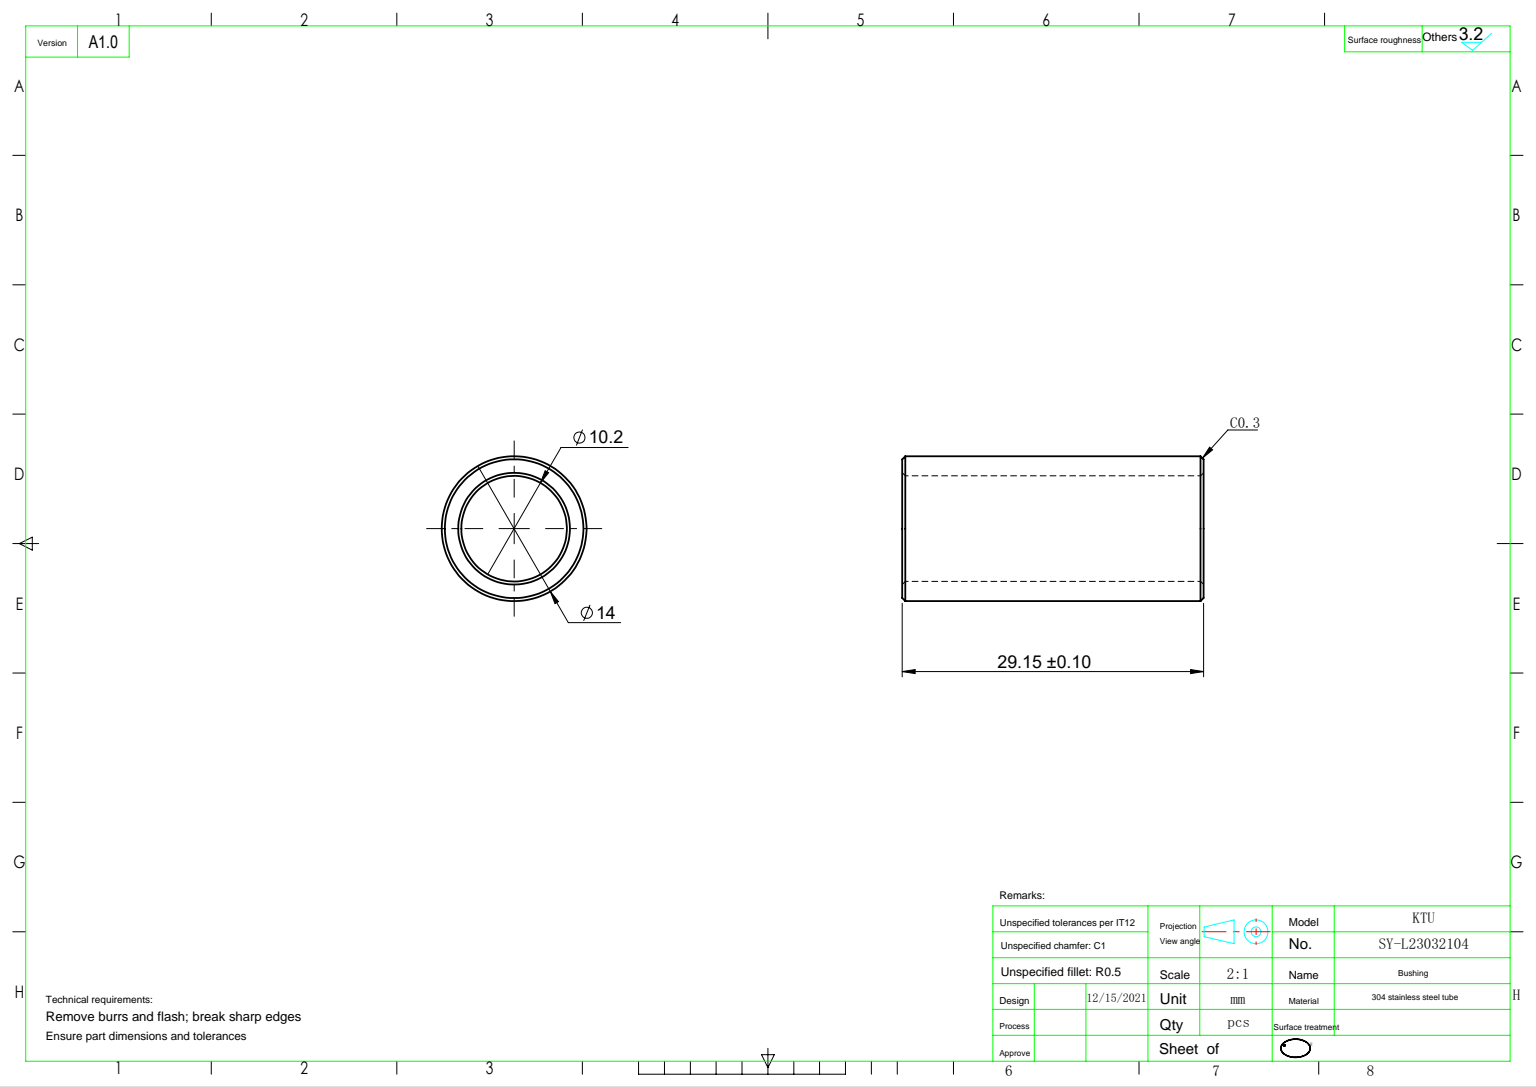
from build123d import *

# Parameters (mm, degrees)
SKETCH_1_R      = 7
SKETCH_1_R_2    = 5.1
EXTRUDE_1_DEPTH = 29.15
CHAMFER_1_SIZE  = 0.3
CHAMFER_2_SIZE  = 0.3


with BuildPart() as part:
    # 草图1 → 凸台-拉伸1 (new body)
    with BuildSketch(Plane.XY):
        Circle(SKETCH_1_R)
        Circle(SKETCH_1_R_2, mode=Mode.SUBTRACT)
    extrude(amount=EXTRUDE_1_DEPTH)

    # 倒角1
    chamfer_1_edges = [part.edges().sort_by_distance(p)[0] for p in [
        (-7, 0, 0),
    ]]
    chamfer(chamfer_1_edges, length=CHAMFER_1_SIZE)

    # 倒角2
    chamfer_2_edges = [part.edges().sort_by_distance(p)[0] for p in [
        (-7, 0, 29.15),
        (-5.1, 0, 0),
        (-5.1, 0, 29.15),
    ]]
    chamfer(chamfer_2_edges, length=CHAMFER_2_SIZE)


solid = part.part
